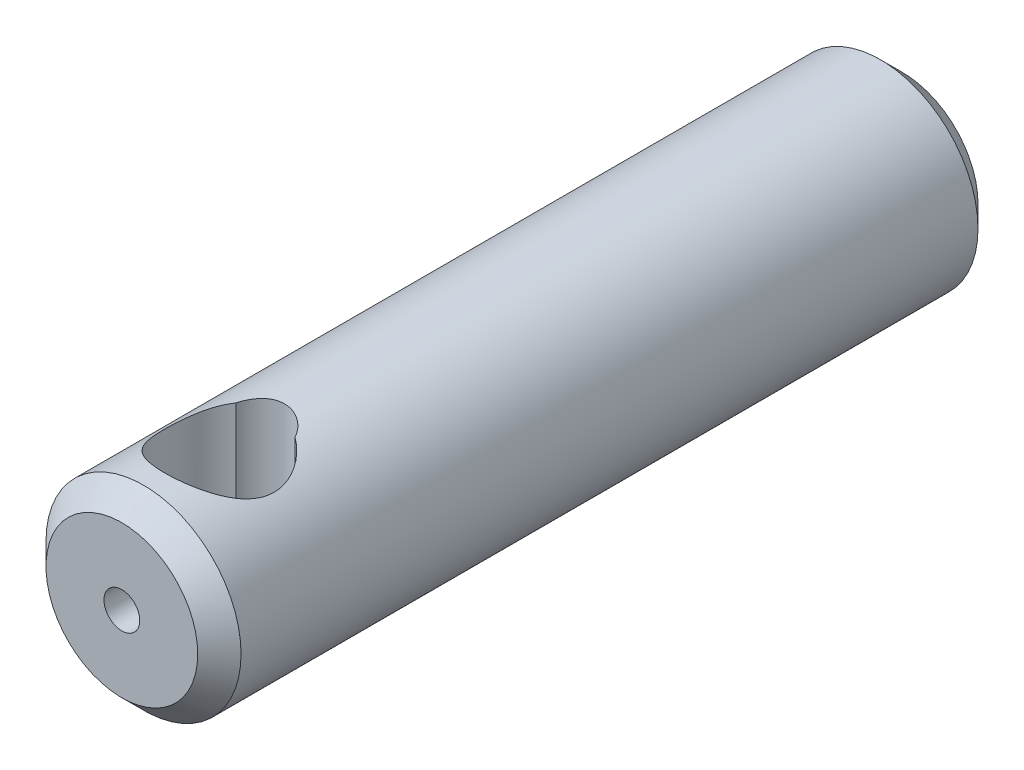
from build123d import *

# Parameters (mm, degrees)
SKETCH1_R               = 9
BOSS_EXTRUDE1_DEPTH     = 72
CUT_EXTRUDE1_DEPTH      = 74.116345642
CUT_EXTRUDE1_DEPTH_BACK = 74.116345642
M4_TAPPED_HOLE1_REACH   = 75.116
M4_TAPPED_HOLE1_BORE_R  = 1.65
CHAMFER1_SIZE           = 2


with BuildPart() as part:
    # Sketch1 → Boss-Extrude1 (new body)
    with BuildSketch(Plane.XY):
        Circle(SKETCH1_R)
    extrude(amount=BOSS_EXTRUDE1_DEPTH)

    # Sketch2 → Cut-Extrude1 (cut, two sides: drawn at the far end of the back side and taken through both)
    with BuildSketch(Plane(origin=(0, 0, 0), x_dir=(1, 0, 0), z_dir=(0, 1, 0)).offset(-CUT_EXTRUDE1_DEPTH_BACK)):
        with BuildLine():
            ThreePointArc((-2.726987011, -58.749583333), (0, -68.05), (2.726987011, -58.749583333))
            ThreePointArc((2.726987011, -58.749583333), (0, -57), (-2.726987011, -58.749583333))
        make_face()
    extrude(amount=CUT_EXTRUDE1_DEPTH + CUT_EXTRUDE1_DEPTH_BACK, mode=Mode.SUBTRACT)

    # M4 Tapped Hole1 bore → M4 Tapped Hole1 (cut, up to next)
    with BuildSketch(Plane.XY.offset(72), mode=Mode.PRIVATE) as m4_tapped_hole1_sk1:
        Circle(M4_TAPPED_HOLE1_BORE_R)
    m4_tapped_hole1_tool1 = extrude(m4_tapped_hole1_sk1.sketch, amount=-M4_TAPPED_HOLE1_REACH, mode=Mode.PRIVATE) & part.part
    add(m4_tapped_hole1_tool1.solids().sort_by_distance((0, 0, 72))[0], mode=Mode.SUBTRACT)

    # Chamfer1
    chamfer1_edges = [part.edges().sort_by_distance(p)[0] for p in [
        (-9, 0, 0),
        (-9, 0, 72),
    ]]
    chamfer(chamfer1_edges, length=CHAMFER1_SIZE)


solid = part.part
